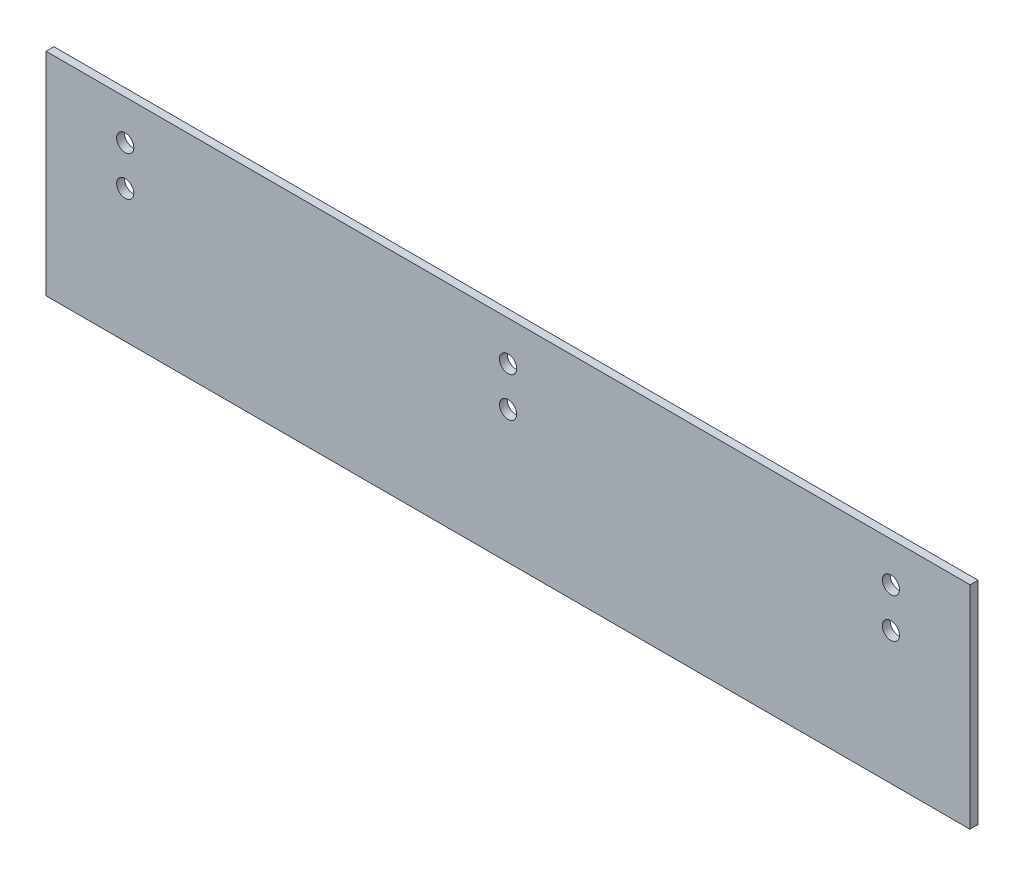
from build123d import *

# Parameters (mm, degrees)
SKETCH_1_W          = 350
SKETCH_1_H          = 85
SKETCH_1_R          = 3.25
EXTRUDE_1_DEPTH     = 3
SKETCH_2_R          = 16.85
CUT_EXTRUDE_1_DEPTH = 366


with BuildPart() as part:
    # 草图1 → 凸台-拉伸1 (new body)
    with BuildSketch(Plane.XY):
        Rectangle(SKETCH_1_W, SKETCH_1_H)
        with Locations((-145, 27.5)):
            Circle(SKETCH_1_R, mode=Mode.SUBTRACT)
        with Locations((-145, 12.5)):
            Circle(SKETCH_1_R, mode=Mode.SUBTRACT)
        with Locations((0, 27.5)):
            Circle(SKETCH_1_R, mode=Mode.SUBTRACT)
        with Locations((0, 12.5)):
            Circle(SKETCH_1_R, mode=Mode.SUBTRACT)
        with Locations((145, 27.5)):
            Circle(SKETCH_1_R, mode=Mode.SUBTRACT)
        with Locations((145, 12.5)):
            Circle(SKETCH_1_R, mode=Mode.SUBTRACT)
    extrude(amount=EXTRUDE_1_DEPTH)

    # 草图2 → 切除-拉伸1 (cut)
    with BuildSketch(Plane(origin=(175, 0, 0), x_dir=(0, 0, -1), z_dir=(1, 0, 0))):
        with Locations((-1.5, -54.5)):
            Circle(SKETCH_2_R)
    extrude(amount=-CUT_EXTRUDE_1_DEPTH, mode=Mode.SUBTRACT)


solid = part.part
